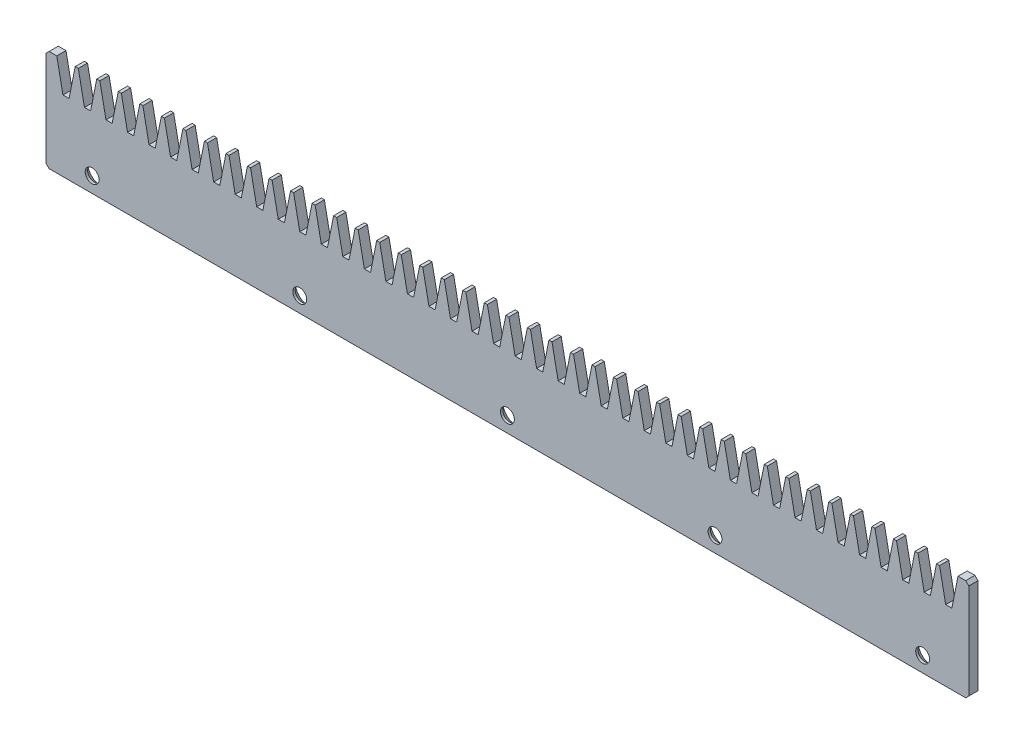
SolidWorks part; units mm, degrees
material "SUS304"
ref_plane "前视基准面" through (0, 0, 0) normal (0, 0, 1) x (1, 0, 0)
ref_plane "上视基准面" through (0, 0, 0) normal (0, 1, 0) x (1, 0, 0)
ref_plane "右视基准面" through (0, 0, 0) normal (1, 0, 0) x (0, 0, -1)
sketch "草图2" plane through (0, 0, 0) normal (0, 0, 1) x (1, 0, 0)
  line L1 (0, 0) -> (300, 0)
  line L2 (0, 0) -> (0, 33)
  line L3 (0, 33) -> (300, 33)
  line L4 (300, 0) -> (300, 33)
  dimension "D1" = 33
  dimension "D2" = 300
extrude "凸台-拉伸1" add sketch "草图2" along normal blind 3
sketch "草图3" plane through (0, 0, 3) normal (0, 0, 1) x (1, 0, 0)
  line L9 (3.5, 33) -> (9.5, 33)
  line L11 (300, 33) -> (0, 33) construction
  line L12 (9.5, 33) -> (7.5, 23)
  line L13 (7.5, 23) -> (5.5, 23)
  line L14 (5.5, 23) -> (3.5, 33)
  line L15 (6.5, 23) -> (6.5, 33) construction
  line L17 (12.5, 23) -> (10.5, 33)
  line L18 (16.5, 33) -> (14.5, 23)
  line L19 (10.5, 33) -> (16.5, 33)
  line L20 (14.5, 23) -> (12.5, 23)
  line L21 (19.5, 23) -> (17.5, 33)
  line L22 (23.5, 33) -> (21.5, 23)
  line L23 (17.5, 33) -> (23.5, 33)
  line L24 (21.5, 23) -> (19.5, 23)
  line L25 (26.5, 23) -> (24.5, 33)
  line L26 (30.5, 33) -> (28.5, 23)
  line L27 (24.5, 33) -> (30.5, 33)
  line L28 (28.5, 23) -> (26.5, 23)
  line L29 (33.5, 23) -> (31.5, 33)
  line L30 (37.5, 33) -> (35.5, 23)
  line L31 (31.5, 33) -> (37.5, 33)
  line L32 (35.5, 23) -> (33.5, 23)
  line L33 (40.5, 23) -> (38.5, 33)
  line L34 (44.5, 33) -> (42.5, 23)
  line L35 (38.5, 33) -> (44.5, 33)
  line L36 (42.5, 23) -> (40.5, 23)
  line L37 (47.5, 23) -> (45.5, 33)
  line L38 (51.5, 33) -> (49.5, 23)
  line L39 (45.5, 33) -> (51.5, 33)
  line L40 (49.5, 23) -> (47.5, 23)
  line L41 (54.5, 23) -> (52.5, 33)
  line L42 (58.5, 33) -> (56.5, 23)
  line L43 (52.5, 33) -> (58.5, 33)
  line L44 (56.5, 23) -> (54.5, 23)
  line L45 (61.5, 23) -> (59.5, 33)
  line L46 (65.5, 33) -> (63.5, 23)
  line L47 (59.5, 33) -> (65.5, 33)
  line L48 (63.5, 23) -> (61.5, 23)
  line L49 (68.5, 23) -> (66.5, 33)
  line L50 (72.5, 33) -> (70.5, 23)
  line L51 (66.5, 33) -> (72.5, 33)
  line L52 (70.5, 23) -> (68.5, 23)
  line L53 (75.5, 23) -> (73.5, 33)
  line L54 (79.5, 33) -> (77.5, 23)
  line L55 (73.5, 33) -> (79.5, 33)
  line L56 (77.5, 23) -> (75.5, 23)
  line L57 (82.5, 23) -> (80.5, 33)
  line L58 (86.5, 33) -> (84.5, 23)
  line L59 (80.5, 33) -> (86.5, 33)
  line L60 (84.5, 23) -> (82.5, 23)
  line L61 (89.5, 23) -> (87.5, 33)
  line L62 (93.5, 33) -> (91.5, 23)
  line L63 (87.5, 33) -> (93.5, 33)
  line L64 (91.5, 23) -> (89.5, 23)
  line L65 (96.5, 23) -> (94.5, 33)
  line L66 (100.5, 33) -> (98.5, 23)
  line L67 (94.5, 33) -> (100.5, 33)
  line L68 (98.5, 23) -> (96.5, 23)
  line L69 (103.5, 23) -> (101.5, 33)
  line L70 (107.5, 33) -> (105.5, 23)
  line L71 (101.5, 33) -> (107.5, 33)
  line L72 (105.5, 23) -> (103.5, 23)
  line L73 (110.5, 23) -> (108.5, 33)
  line L74 (114.5, 33) -> (112.5, 23)
  line L75 (108.5, 33) -> (114.5, 33)
  line L76 (112.5, 23) -> (110.5, 23)
  line L77 (117.5, 23) -> (115.5, 33)
  line L78 (121.5, 33) -> (119.5, 23)
  line L79 (115.5, 33) -> (121.5, 33)
  line L80 (119.5, 23) -> (117.5, 23)
  line L81 (124.5, 23) -> (122.5, 33)
  line L82 (128.5, 33) -> (126.5, 23)
  line L83 (122.5, 33) -> (128.5, 33)
  line L84 (126.5, 23) -> (124.5, 23)
  line L85 (131.5, 23) -> (129.5, 33)
  line L86 (135.5, 33) -> (133.5, 23)
  line L87 (129.5, 33) -> (135.5, 33)
  line L88 (133.5, 23) -> (131.5, 23)
  line L89 (138.5, 23) -> (136.5, 33)
  line L90 (142.5, 33) -> (140.5, 23)
  line L91 (136.5, 33) -> (142.5, 33)
  line L92 (140.5, 23) -> (138.5, 23)
  line L141 (3.5, 33) -> (226.5, 33) construction
  line L142 (145.5, 23) -> (143.5, 33)
  line L143 (149.5, 33) -> (147.5, 23)
  line L144 (143.5, 33) -> (149.5, 33)
  line L145 (147.5, 23) -> (145.5, 23)
  line L146 (152.5, 23) -> (150.5, 33)
  line L147 (156.5, 33) -> (154.5, 23)
  line L148 (150.5, 33) -> (156.5, 33)
  line L149 (154.5, 23) -> (152.5, 23)
  line L150 (159.5, 23) -> (157.5, 33)
  line L151 (163.5, 33) -> (161.5, 23)
  line L152 (157.5, 33) -> (163.5, 33)
  line L153 (161.5, 23) -> (159.5, 23)
  line L154 (166.5, 23) -> (164.5, 33)
  line L155 (170.5, 33) -> (168.5, 23)
  line L156 (164.5, 33) -> (170.5, 33)
  line L157 (168.5, 23) -> (166.5, 23)
  line L158 (173.5, 23) -> (171.5, 33)
  line L159 (177.5, 33) -> (175.5, 23)
  line L160 (171.5, 33) -> (177.5, 33)
  line L161 (175.5, 23) -> (173.5, 23)
  line L166 (180.5, 23) -> (178.5, 33)
  line L167 (184.5, 33) -> (182.5, 23)
  line L168 (178.5, 33) -> (184.5, 33)
  line L169 (182.5, 23) -> (180.5, 23)
  line L170 (187.5, 23) -> (185.5, 33)
  line L171 (191.5, 33) -> (189.5, 23)
  line L172 (185.5, 33) -> (191.5, 33)
  line L173 (189.5, 23) -> (187.5, 23)
  line L174 (194.5, 23) -> (192.5, 33)
  line L175 (198.5, 33) -> (196.5, 23)
  line L176 (192.5, 33) -> (198.5, 33)
  line L177 (196.5, 23) -> (194.5, 23)
  line L178 (201.5, 23) -> (199.5, 33)
  line L179 (205.5, 33) -> (203.5, 23)
  line L180 (199.5, 33) -> (205.5, 33)
  line L181 (203.5, 23) -> (201.5, 23)
  line L182 (208.5, 23) -> (206.5, 33)
  line L183 (212.5, 33) -> (210.5, 23)
  line L184 (206.5, 33) -> (212.5, 33)
  line L185 (210.5, 23) -> (208.5, 23)
  line L186 (215.5, 23) -> (213.5, 33)
  line L187 (219.5, 33) -> (217.5, 23)
  line L188 (213.5, 33) -> (219.5, 33)
  line L189 (217.5, 23) -> (215.5, 23)
  line L190 (222.5, 23) -> (220.5, 33)
  line L191 (226.5, 33) -> (224.5, 23)
  line L192 (220.5, 33) -> (226.5, 33)
  line L193 (224.5, 23) -> (222.5, 23)
  line L194 (229.5, 23) -> (227.5, 33)
  line L195 (233.5, 33) -> (231.5, 23)
  line L196 (227.5, 33) -> (233.5, 33)
  line L197 (231.5, 23) -> (229.5, 23)
  line L198 (236.5, 23) -> (234.5, 33)
  line L199 (240.5, 33) -> (238.5, 23)
  line L200 (234.5, 33) -> (240.5, 33)
  line L201 (238.5, 23) -> (236.5, 23)
  line L202 (243.5, 23) -> (241.5, 33)
  line L203 (247.5, 33) -> (245.5, 23)
  line L204 (241.5, 33) -> (247.5, 33)
  line L205 (245.5, 23) -> (243.5, 23)
  line L206 (250.5, 23) -> (248.5, 33)
  line L207 (254.5, 33) -> (252.5, 23)
  line L208 (248.5, 33) -> (254.5, 33)
  line L209 (252.5, 23) -> (250.5, 23)
  line L210 (257.5, 23) -> (255.5, 33)
  line L211 (261.5, 33) -> (259.5, 23)
  line L212 (255.5, 33) -> (261.5, 33)
  line L213 (259.5, 23) -> (257.5, 23)
  line L214 (264.5, 23) -> (262.5, 33)
  line L215 (268.5, 33) -> (266.5, 23)
  line L216 (262.5, 33) -> (268.5, 33)
  line L217 (266.5, 23) -> (264.5, 23)
  line L218 (271.5, 23) -> (269.5, 33)
  line L219 (275.5, 33) -> (273.5, 23)
  line L220 (269.5, 33) -> (275.5, 33)
  line L221 (273.5, 23) -> (271.5, 23)
  line L222 (278.5, 23) -> (276.5, 33)
  line L223 (282.5, 33) -> (280.5, 23)
  line L224 (276.5, 33) -> (282.5, 33)
  line L225 (280.5, 23) -> (278.5, 23)
  line L226 (285.5, 23) -> (283.5, 33)
  line L227 (289.5, 33) -> (287.5, 23)
  line L228 (283.5, 33) -> (289.5, 33)
  line L229 (287.5, 23) -> (285.5, 23)
  line L230 (292.5, 23) -> (290.5, 33)
  line L231 (296.5, 33) -> (294.5, 23)
  line L232 (290.5, 33) -> (296.5, 33)
  line L233 (294.5, 23) -> (292.5, 23)
  line L234 (5.5, 23) -> (294.5, 23) construction
  line L235 (150, 23) -> (150, 0) construction
  line L236 (0, 0) -> (300, 0) construction
  dimension "D1" = 6
  dimension "D2" = 10
  dimension "D3" = 2
  dimension "D4" = 7
  dimension "D5" = 42
extrude "切除-拉伸1" cut sketch "草图3" against normal blind 15
chamfer "倒角1" distance 1 angle 45 4 edges at (300, 0, 1.5) (300, 33, 1.5) (0, 0, 1.5) (0, 33, 1.5)
hole_wizard "M4 六角凹锥坑螺钉的锥形沉头孔1" positions "草图4" profile "草图5" countersink size "M4" standard "ISO"
sketch "草图4" plane through (0, 0, 0) normal (0, 0, -1) x (-1, 0, 0)
  line L0 (-1, 0) -> (-299, 0) construction
  line L1 (-300, 1) -> (-300, 32) construction
  line L2 (-285, 5) -> (-15, 5) construction
  line L4 (-150, 5) -> (-150, 0) construction
  point P0 (-285, 5)
  point P8 (-217.5, 5)
  point P9 (-150, 5)
  point P10 (-82.5, 5)
  point P11 (-15, 5)
  dimension "D2" = 5
  dimension "D3" = 15
  dimension "D1" = 5
sketch "草图5" plane through (285, 5, 0) normal (1, 0, 0) x (0, 1, 0)
  line L0 (0, 0) -> (0, 12.8519)
  line L1 (0, 12.8519) -> (2.25, 11.5)
  line L2 (2.25, 11.5) -> (2.25, 2.23)
  line L3 (2.25, 2.23) -> (4.48, 0)
  line L5 (4.48, 0) -> (0, 0)
  line L6 (-2.25, 2.23) -> (-4.48, 0) construction
  line L10 (0, 12.8519) -> (-2.25, 11.5) construction
  line L11 (0, -6.35) -> (0, 107.95) construction
  dimension "孔直径" = 4.5
  dimension "孔深度" = 11.5
  dimension "近端锥形沉头孔直径" = 8.96
  dimension "近端锥形沉头孔角度" = 90
  dimension "导头角度" = 118
